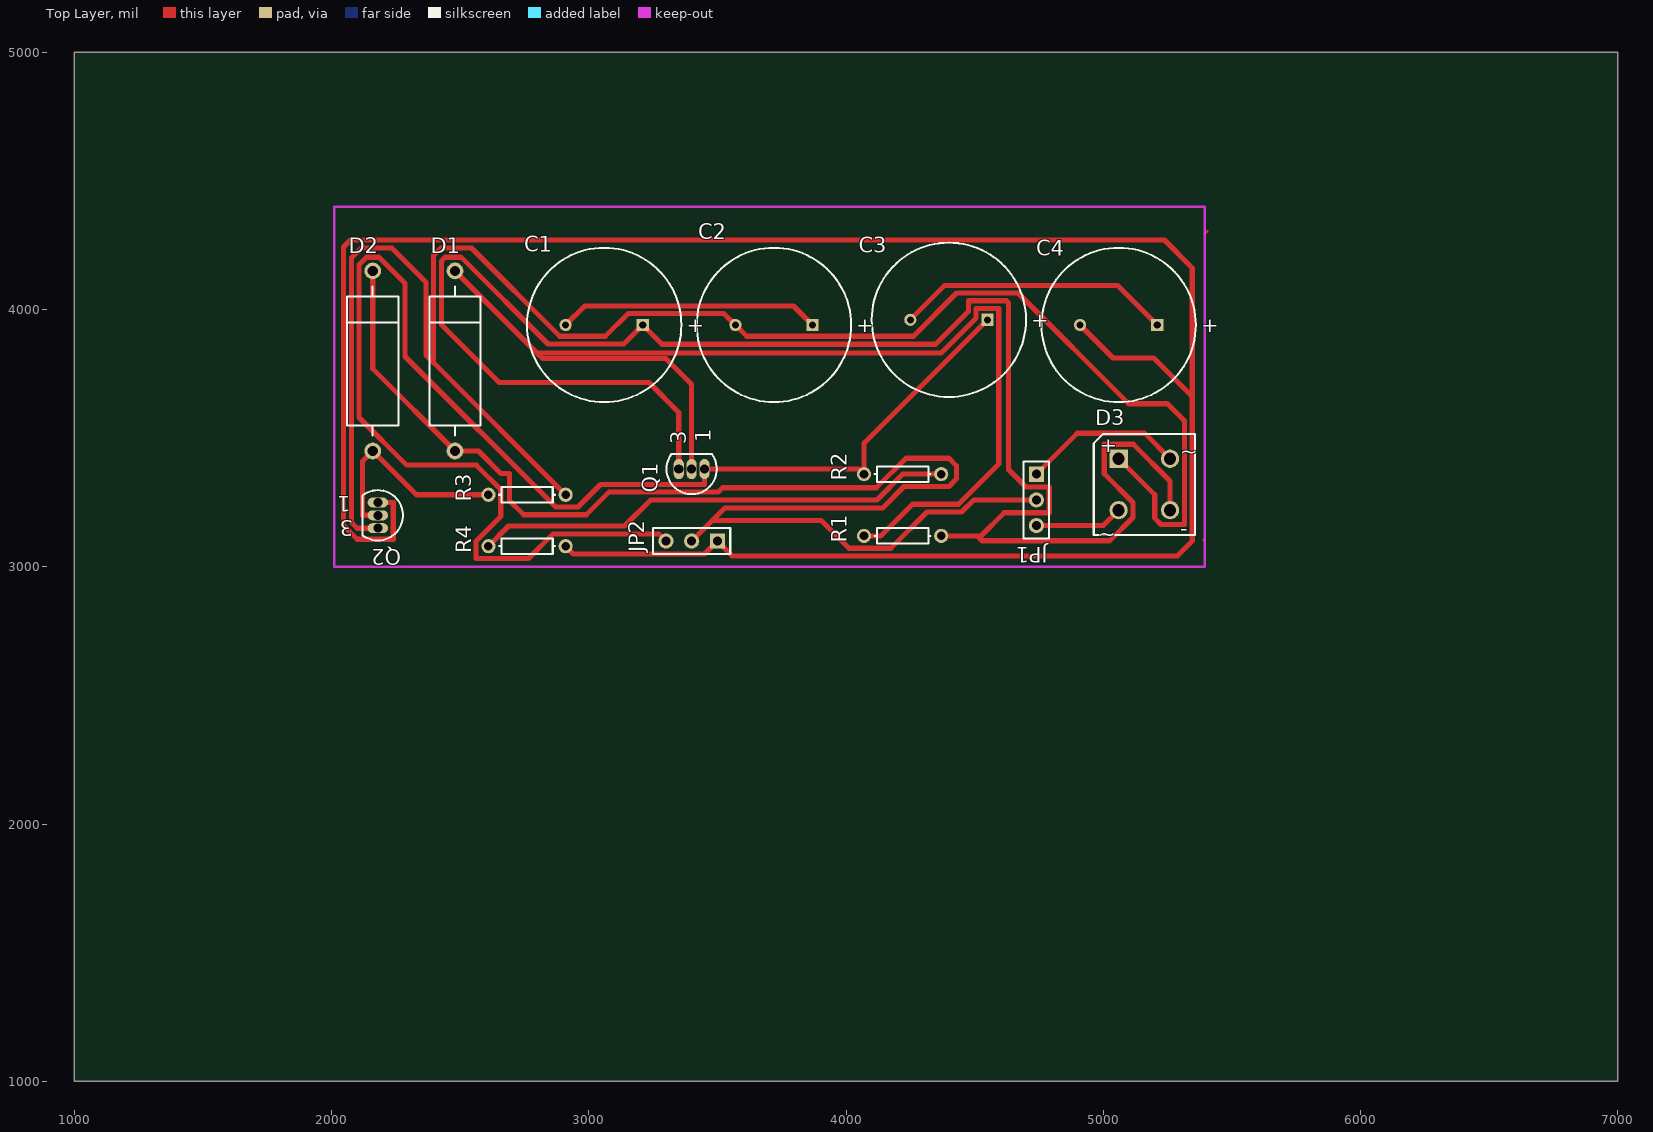
[diagram p0: Top Layer view]
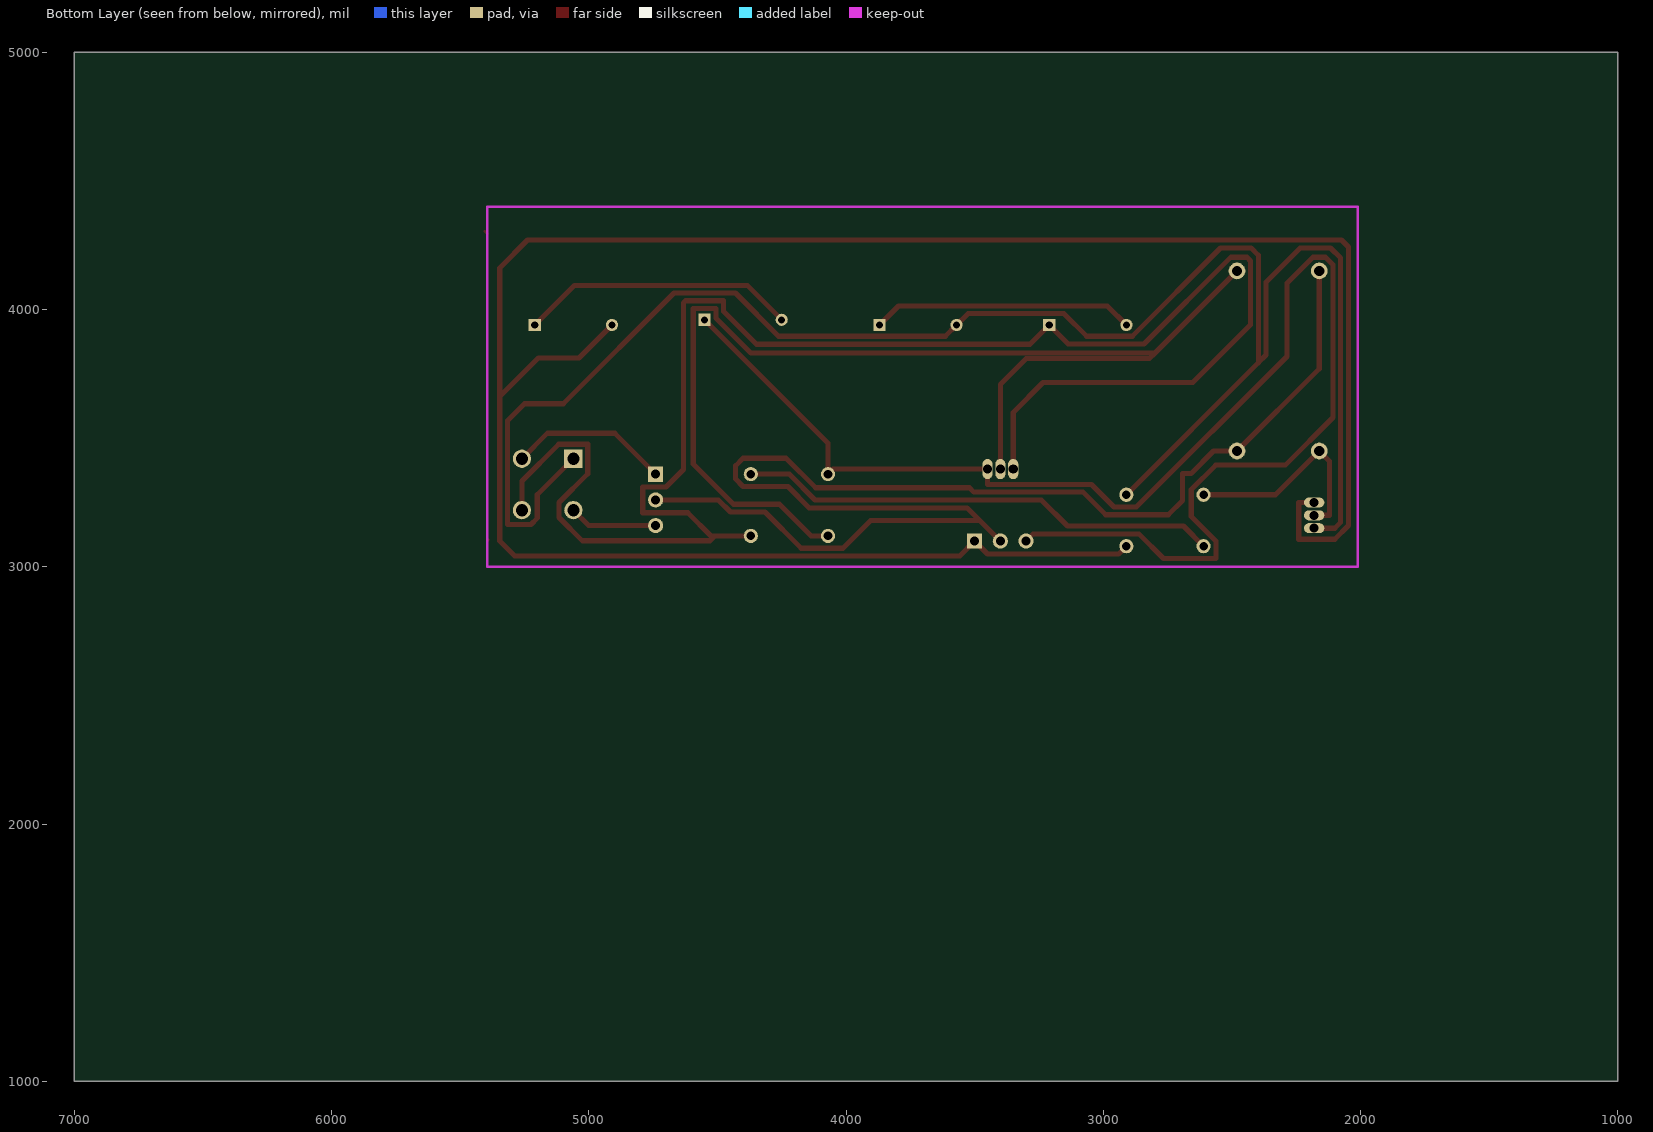
[diagram p1: Bottom Layer view, seen from below]
# Altium PCB MISC95138.PCBDOC
Units mil, origin at the board's own origin, x right, y up, seen from the top; angles counter-clockwise.
Board outline 6000 x 4000 mil, 2 copper layers (Top Layer, Bottom Layer); 15 components, 12 nets, 36 pads, 0 vias.

## Layer stack, top to bottom (the 12.6 mil dielectric is the usual default, probably not edited)
Top Layer: signal copper 1.4
Dielectric: dielectric 12.6, FR-4, Dk 4.8
Bottom Layer: signal copper 1.4

## Board outline
1000,1000 7000,1000 7000,5000 1000,5000

## Design rules (kind name [scope] priority, off if disabled: settings)
Clearance [All] p1: gap=10
ComponentClearance [All] p1: gap=10 collisioncheckmode=0
PolygonConnect [All] p1: connectstyle=Relief reliefconductorwidth=10 reliefentries=4 polygonreliefangle="90 Angle"
RoutingLayers buxian [All] p1: top layer=Horizontal bottom layer=Vertical // rules for zhengfudianyuan
RoutingLayers [All] p2: top layer=Horizontal bottom layer=Vertical
RoutingVias [All] p1: holewidth=28 width=50 viastyle="Through Hole" minholewidth=28 minwidth=50 maxholewidth=28 maxwidth=50
SolderMaskExpansion [All] p1: expansion=4
TestPointUsage [All] p1: valid=0 allowmultiple=FALSE
Testpoint [All] p1: side=15 testpointundercomponent=TRUE minsize=40 maxsize=100 preferedsize=60 minholesize=0 maxholesize=40 preferedholesize=32 testpointgrid=1 style=1023 order=1234567890
Width "Width Rules" [All] p1: maxlimit=20 minlimit=20 preferedwidth=20
16 further rules are at their usual default settings.

## Components (designator, comment, footprint, x,y, rotation, side; value= is the part's Value field where it differs from the comment)
C1 "Cap Pol1" RB7.6-15 3060,3940 r0 top
C2 "Cap Pol1" RB7.6-15 3720,3940 r0 top
C3 "Cap Pol1" RB7.6-15 4400,3960 r0 top
C4 "Cap Pol1" RB7.6-15 5060,3940 r0 top
D1 "IN4736" DIODE-0.7 2480,3800 r90 top
D2 "IN4736" DIODE-0.7 2160,3800 r90 top
D3 "Bridge1" E-BIP-P4/D10 5160,3320 r0 top
JP1 "Header 3" HDR1X3 4740,3360 r270 top
JP2 "Header 3" HDR1X3 3500,3100 r180 top
Q1 "2N3904" BCY-W3/E4 3400,3380 r90 top
Q2 "2N3906" BCY-W3/E4 2180,3200 r180 top
R1 "Res1" AXIAL-0.3 4220,3120 r180 top
R2 "Res1" AXIAL-0.3 4220,3360 r180 top
R3 "Res1" AXIAL-0.3 2760,3280 r180 top
R4 "Res1" AXIAL-0.3 2760,3080 r180 top

## Footprints (in the part's own frame and the unit in brackets; to place one, negate y for a bottom-side part, rotate by r counter-clockwise, add the part's x,y. Pads: shape width x height; smd on the part's side, far side on the other; paste and mask are expansions set on the pad)
AXIAL-0.3 [mm]
  round 1.4 hole 0.85: 1(-3.81,0) 2(3.81,0)
  silkscreen extent -2.77,-0.76 2.77,0.76
BCY-W3/E4 [mm]
  oval 2x1 hole 0.9: 1(0,-1.27) 2(0,0) 3(0,1.27)
  silkscreen extent -2.48,-2.48 1.5,2.48
DIODE-0.7 [mm]
  round 1.65 hole 1: 1(-8.89,0) 2(8.89,0)
  silkscreen extent -7.37,-2.54 7.37,2.54
E-BIP-P4/D10 [mm]
  rect 1.8x1.8 hole 1.2: 1(-2.54,2.54)
  round 1.8 hole 1.2: 2(-2.54,-2.54) 3(2.54,-2.54) 4(2.54,2.54)
  silkscreen extent -5,-5 5,5
HDR1X3 [mm] "Connector; Header; 3 Position"
  rect 1.5x1.5 hole 0.9: 1(0,0)
  round 1.5 hole 0.9: 2(2.54,0) 3(5.08,0)
  silkscreen extent -1.27,-1.27 6.35,1.27
RB7.6-15 [mm]
  rect 1.2x1.2 hole 0.7: 1(3.81,0)
  round 1.2 hole 0.7: 2(-3.81,0)
  silkscreen extent -7.62,-7.62 7.62,7.62

## Part data
C1 C2 C3 C4: "Polarized Capacitor (Radial)"
D1 D2: library part "D Zener", "Zener Diode"
D3: "Full Wave Diode Bridge"
JP1 JP2: "Header, 3-Pin"
Q1: "NPN General Purpose Amplifier"
Q2: "PNP General Purpose Amplifier"
R1 R2 R3 R4: "Resistor"

## Nets (pads, with @x,y where several pads share a name; then routed paths per layer and width w, separated by ;. In a path a pad name is that pad's centre, name@x,y a point inside that pad or via, vN(x,y) a via of type N, cw(c..) or ccw(c..) an arc to the next point about the centre after c; other vN are vias at no path point)
GND: D1.1 D2.2 JP1.2 JP2.2 | length 5612.4
  Top Layer w20: D2.2 2160,3770 D1.1 2571,3450 2659,3362 2692,3362 2692,3257 2747,3202 2990,3202 3078,3290 3503,3290 3520,3307 4118,3307 4233,3422 4400,3422 4429,3393 4429,3341 4400,3312 4226,3312 4143,3229 3529,3229 3480,3180 ; JP2.2 3480,3180 ; JP1.2 4496.43,3260 4449.43,3213 4315,3213 4174,3072 4012,3072 3904,3180 3480,3180
NetC1_1: C1.1 D3.3 Q1.3 R1.1 | length 6843.3
  Top Layer w20: Q1.3 3350,3600 3234,3716 2652,3716 2427,3941 2427,4189 2441,4203 2504,4203 2841,3866 3136,3866 C1.1 3285,3865 4348,3865 4476,3993 4476,4034 4624,4034 4632,4026 4632,3378 4700,3310 4790,3310 4790,3210 4615,3210 4525,3120 4510,3120 ; R1.1 4510,3120 ; D3.3 5260,3333 5117,3476 5004,3476 5004,3361.43 5116,3249.43 5116,3192 5025,3101 4529,3101 4510,3120
NetC1_2: C1.2 C2.1 | length 1021.3
  Top Layer w20: C1.2 2984,4014 3796,4014 C2.1
NetC2_2: C2.2 D3.1 Q2.3 R3.1 | length 7209.6
  Top Layer w20: Q2.3 2100,3150 2077,3173 2077,4200 2116,4239 2234,4239 2367,4106 2367,3823 2397,3793 ; R3.1 2397,3793 ; D3.1 5200,3280 5200,3189 5225,3164 5316,3164 5316,3568 5250,3634 5099,3634 4669,4064 4430,4064 4262,3896 3614,3896 C2.2 3526,3984 3152,3984 3064,3896 2887,3896 2544,4239 2425,4239 2397,4211 2397,3793
NetC3_1: C3.1 JP2.3 Q1.1 R2.2 | length 5805.4
  Top Layer w20: JP2.3 3272,3128 2862,3128 2766,3032 2562,3032 2562,3099.56 2658,3195.56 2658,3300 2563,3395 2292.48,3395 2107,3580.48 2107,4174.48 2135.52,4203 2185,4203 2286,4102 2286,3817.72 2871.72,3232 2958,3232 3046,3320 3450,3320 Q1.1 4050,3380 R2.2 4070,3480 C3.1
NetC3_2: C3.2 C4.1 | length 1079.3
  Top Layer w20: C3.2 4384,4094 5056,4094 C4.1
NetC4_2: C4.2 JP2.1 Q2.1 R4.1 | length 8986.2
  Top Layer w20: Q2.1 2240,3250 2240,3107 2100,3107 2047,3160 2047,4243 2074,4270 5238,4270 5346,4162 5346,3662 ; R4.1 2940,3050 3450,3050 JP2.1 3558,3042 5288,3042 5346,3100 5346,3662 ; C4.2 5038,3812 5196,3812 5346,3662
NetD1_2: D1.2 Q1.2 R1.2 | length 4564
  Top Layer w20: D1.2 2799,3831 ; Q1.2 3400,3709 3300,3809 2821,3809 2799,3831 ; R1.2 4135,3120 4258,3243 4437,3243 4594,3400 4594,4004 4506,4004 4506,3967 4370,3831 2799,3831
NetD2_1: D2.1 Q2.2 R3.2 | length 847
  Top Layer w20: Q2.2 2120,3200 2120,3410 D2.1 2330,3280 R3.2
NetD3_2: D3.2 JP1.3 | length 344.9
  Top Layer w20: JP1.3 5000,3160 D3.2
NetD3_4: D3.4 JP1.1 | length 626.9
  Top Layer w20: JP1.1 4899,3519 5161,3519 D3.4
NetR2_1: R2.1 R4.2 | length 1876
  Top Layer w20: R4.2 2688,3158 3139,3158 3241,3260 4120,3260 4220,3360 R2.1
copper on no net: | length 21.2
  Top Layer w10: 5390,3105 5395,3100 ; 5395,4295 5405,4305

## Keep-outs
Keep-Out Layer:
  lines w10: 5390,3000 2010,3000 2010,4400 5395,4400 5395,3000